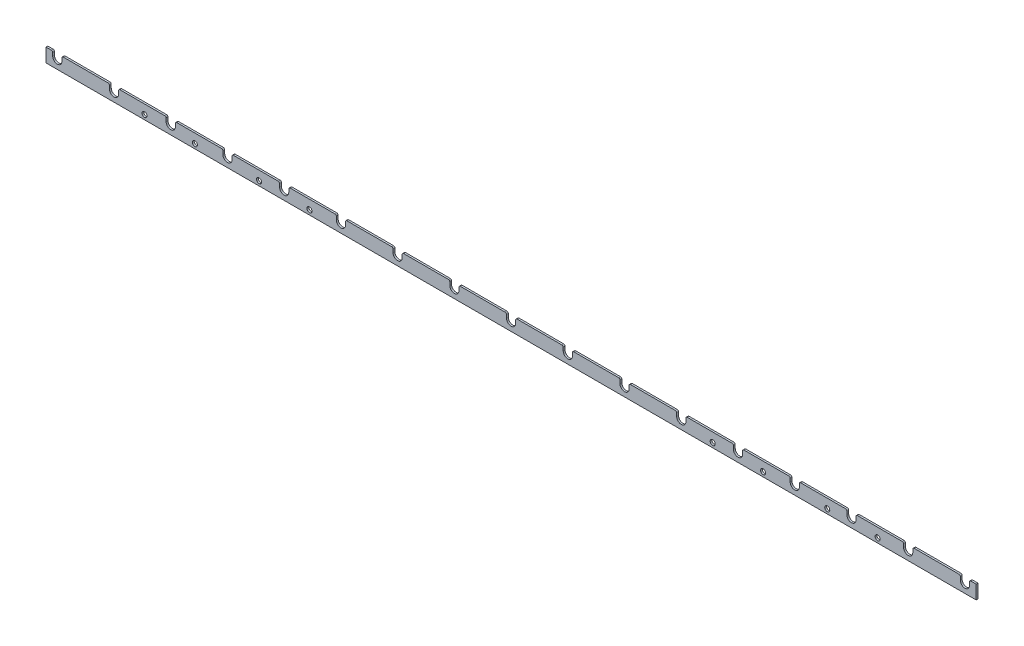
from build123d import *

# Parameters (mm, degrees)
SKETCH_1_W          = 2030
SKETCH_1_H          = 30
EXTRUDE_1_DEPTH     = 4
CUT_EXTRUDE_1_DEPTH = 4
FILLET_1_R          = 3
SKETCH_3_R          = 5.5
CUT_EXTRUDE_2_DEPTH = 4


with BuildPart() as part:
    # 草图1 → 凸台-拉伸1 (new body)
    with BuildSketch(Plane.XY):
        Rectangle(SKETCH_1_W, SKETCH_1_H)
    extrude(amount=EXTRUDE_1_DEPTH)

    # 草图2 → 切除-拉伸1 (cut)
    with BuildSketch(Plane.XY.offset(4)):
        with BuildLine():
            Line((-1000.4, 5), (-1000.4, 15))
            Line((-1000.4, 15), (-980.4, 15))
            Line((-980.4, 15), (-980.4, 5))
            ThreePointArc((-980.4, 5), (-990.4, -5), (-1000.4, 5))
        make_face()
        with BuildLine():
            Line((-856.6, 15), (-876.6, 15))
            Line((-876.6, 15), (-876.6, 5))
            ThreePointArc((-876.6, 5), (-866.6, -5), (-856.6, 5))
            Line((-856.6, 5), (-856.6, 15))
        make_face()
        with BuildLine():
            Line((-732.8, 15), (-752.8, 15))
            Line((-752.8, 15), (-752.8, 5))
            ThreePointArc((-752.8, 5), (-742.8, -5), (-732.8, 5))
            Line((-732.8, 5), (-732.8, 15))
        make_face()
        with BuildLine():
            Line((-609, 15), (-629, 15))
            Line((-629, 15), (-629, 5))
            ThreePointArc((-629, 5), (-619, -5), (-609, 5))
            Line((-609, 5), (-609, 15))
        make_face()
        with BuildLine():
            Line((-485.2, 15), (-505.2, 15))
            Line((-505.2, 15), (-505.2, 5))
            ThreePointArc((-505.2, 5), (-495.2, -5), (-485.2, 5))
            Line((-485.2, 5), (-485.2, 15))
        make_face()
        with BuildLine():
            Line((-361.4, 15), (-381.4, 15))
            Line((-381.4, 15), (-381.4, 5))
            ThreePointArc((-381.4, 5), (-371.4, -5), (-361.4, 5))
            Line((-361.4, 5), (-361.4, 15))
        make_face()
        with BuildLine():
            Line((-237.6, 15), (-257.6, 15))
            Line((-257.6, 15), (-257.6, 5))
            ThreePointArc((-257.6, 5), (-247.6, -5), (-237.6, 5))
            Line((-237.6, 5), (-237.6, 15))
        make_face()
        with BuildLine():
            Line((-113.8, 15), (-133.8, 15))
            Line((-133.8, 15), (-133.8, 5))
            ThreePointArc((-133.8, 5), (-123.8, -5), (-113.8, 5))
            Line((-113.8, 5), (-113.8, 15))
        make_face()
        with BuildLine():
            Line((10, 15), (-10, 15))
            Line((-10, 15), (-10, 5))
            ThreePointArc((-10, 5), (0, -5), (10, 5))
            Line((10, 5), (10, 15))
        make_face()
        with BuildLine():
            Line((133.8, 15), (113.8, 15))
            Line((113.8, 15), (113.8, 5))
            ThreePointArc((113.8, 5), (123.8, -5), (133.8, 5))
            Line((133.8, 5), (133.8, 15))
        make_face()
        with BuildLine():
            Line((257.6, 15), (237.6, 15))
            Line((237.6, 15), (237.6, 5))
            ThreePointArc((237.6, 5), (247.6, -5), (257.6, 5))
            Line((257.6, 5), (257.6, 15))
        make_face()
        with BuildLine():
            Line((381.4, 15), (361.4, 15))
            Line((361.4, 15), (361.4, 5))
            ThreePointArc((361.4, 5), (371.4, -5), (381.4, 5))
            Line((381.4, 5), (381.4, 15))
        make_face()
        with BuildLine():
            Line((505.2, 15), (485.2, 15))
            Line((485.2, 15), (485.2, 5))
            ThreePointArc((485.2, 5), (495.2, -5), (505.2, 5))
            Line((505.2, 5), (505.2, 15))
        make_face()
        with BuildLine():
            Line((629, 15), (609, 15))
            Line((609, 15), (609, 5))
            ThreePointArc((609, 5), (619, -5), (629, 5))
            Line((629, 5), (629, 15))
        make_face()
        with BuildLine():
            Line((752.8, 15), (732.8, 15))
            Line((732.8, 15), (732.8, 5))
            ThreePointArc((732.8, 5), (742.8, -5), (752.8, 5))
            Line((752.8, 5), (752.8, 15))
        make_face()
        with BuildLine():
            Line((876.6, 15), (856.6, 15))
            Line((856.6, 15), (856.6, 5))
            ThreePointArc((856.6, 5), (866.6, -5), (876.6, 5))
            Line((876.6, 5), (876.6, 15))
        make_face()
        with BuildLine():
            Line((1000.4, 15), (980.4, 15))
            Line((980.4, 15), (980.4, 5))
            ThreePointArc((980.4, 5), (990.4, -5), (1000.4, 5))
            Line((1000.4, 5), (1000.4, 15))
        make_face()
    extrude(amount=-CUT_EXTRUDE_1_DEPTH, mode=Mode.SUBTRACT)

    # 圆角1
    fillet_1_edges = [part.edges().sort_by_distance(p)[0] for p in [
        (-876.6, 15, 2),
        (-856.6, 15, 2),
        (-752.8, 15, 2),
        (-732.8, 15, 2),
        (-629, 15, 2),
        (-609, 15, 2),
        (-505.2, 15, 2),
        (-485.2, 15, 2),
        (-381.4, 15, 2),
        (-361.4, 15, 2),
        (-257.6, 15, 2),
        (-237.6, 15, 2),
        (-133.8, 15, 2),
        (-113.8, 15, 2),
        (-10, 15, 2),
        (10, 15, 2),
        (113.8, 15, 2),
        (133.8, 15, 2),
        (237.6, 15, 2),
        (257.6, 15, 2),
        (361.4, 15, 2),
        (381.4, 15, 2),
        (485.2, 15, 2),
        (505.2, 15, 2),
        (609, 15, 2),
        (629, 15, 2),
        (732.8, 15, 2),
        (752.8, 15, 2),
        (856.6, 15, 2),
        (876.6, 15, 2),
        (980.4, 15, 2),
        (1000.4, 15, 2),
        (-1000.4, 15, 2),
        (-980.4, 15, 2),
    ]]
    fillet(fillet_1_edges, radius=FILLET_1_R)

    # 草图3 → 切除-拉伸2 (cut)
    with BuildSketch(Plane.XY.offset(4)):
        with Locations((-800, -5)):
            Circle(SKETCH_3_R)
        with Locations((-690, -5)):
            Circle(SKETCH_3_R)
        with Locations((-550, -5)):
            Circle(SKETCH_3_R)
        with Locations((-440, -5)):
            Circle(SKETCH_3_R)
        with Locations(Location((440, -5, 0), (0, 0, 180))):
            Circle(SKETCH_3_R)
        with Locations(Location((550, -5, 0), (0, 0, 180))):
            Circle(SKETCH_3_R)
        with Locations(Location((690, -5, 0), (0, 0, 180))):
            Circle(SKETCH_3_R)
        with Locations(Location((800, -5, 0), (0, 0, 180))):
            Circle(SKETCH_3_R)
    extrude(amount=-CUT_EXTRUDE_2_DEPTH, mode=Mode.SUBTRACT)


solid = part.part
